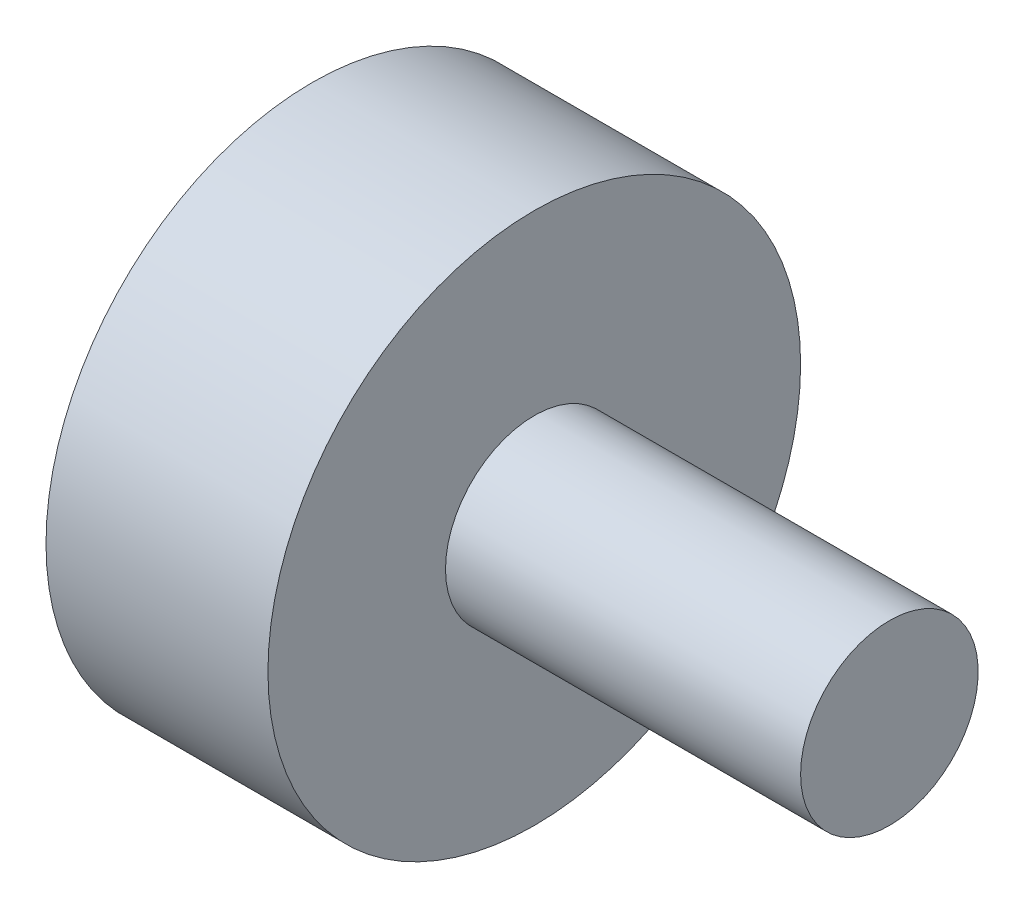
SolidWorks part; units mm, degrees
ref_plane "Front Plane" through (0, 0, 0) normal (0, 0, 1) x (1, 0, 0)
ref_plane "Top Plane" through (0, 0, 0) normal (0, 1, 0) x (1, 0, 0)
ref_plane "Right Plane" through (0, 0, 0) normal (1, 0, 0) x (0, 0, -1)
sketch "Sketch1" plane through (0, 0, 0) normal (0, 0, 1) x (1, 0, 0)
  line L0 (0, 0) -> (51.3633, 0) construction
  line L1 (0, 0) -> (0, 6)
  line L2 (0, 6) -> (5, 6)
  line L3 (5, 6) -> (5, 2)
  line L4 (5, 2) -> (13, 2)
  line L5 (13, 2) -> (13, 0)
  line L6 (0, 0) -> (13, 0)
  dimension "D1" = 5
  dimension "D2" = 8
  dimension "D3" = 2
  dimension "D4" = 6
revolve "Revolve1" add sketch "Sketch1" angle 360 about L0
